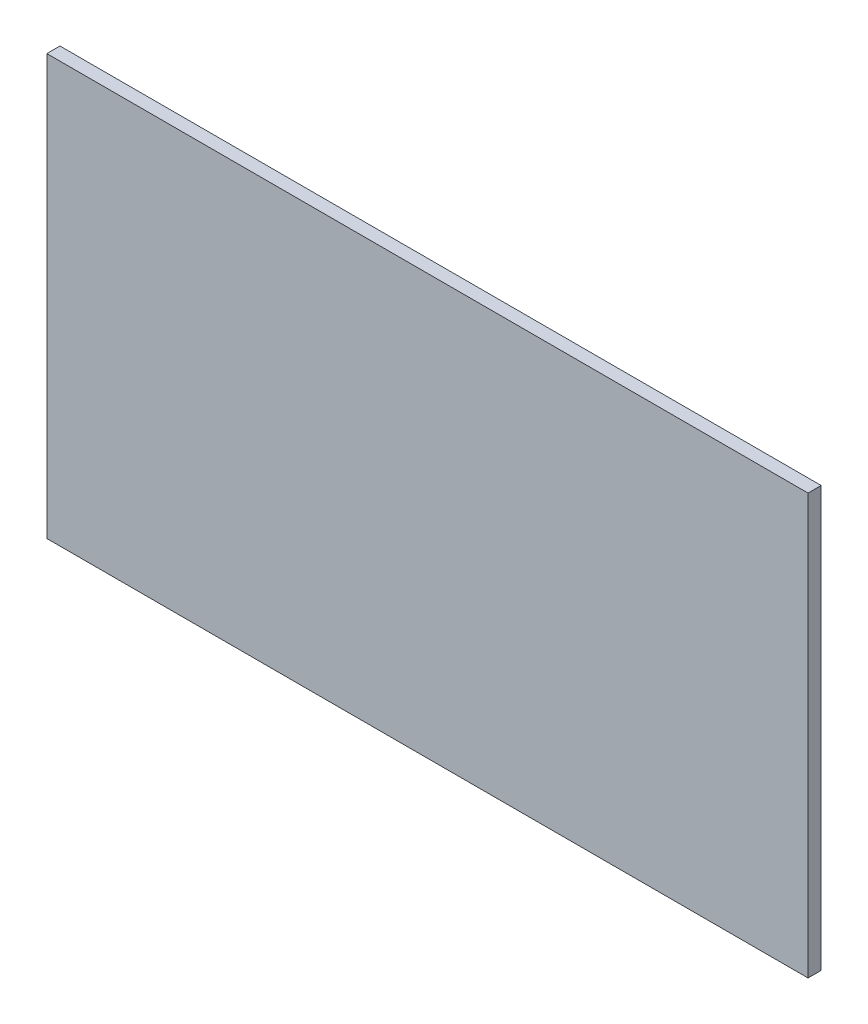
from build123d import *

# Parameters (mm, degrees)
SKETCH_1_W      = 58
SKETCH_1_H      = 32
EXTRUDE_1_DEPTH = 0.5


with BuildPart() as part:
    # 草图1 → 凸台-拉伸1 (new, symmetric)
    with BuildSketch(Plane.XY):
        Rectangle(SKETCH_1_W, SKETCH_1_H)
    extrude(amount=EXTRUDE_1_DEPTH, both=True)


solid = part.part
